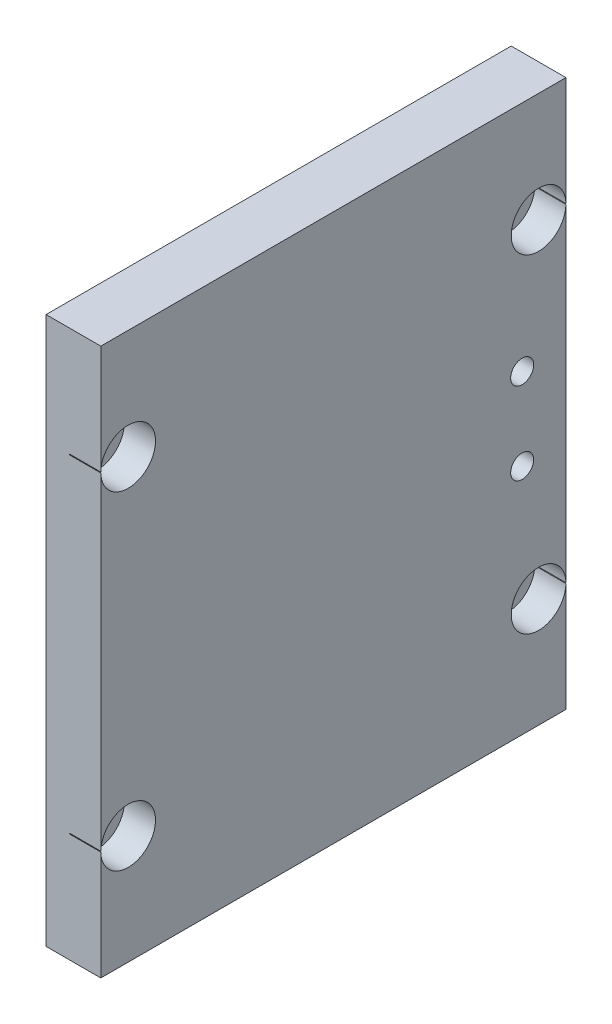
SolidWorks part; units mm, degrees
ref_plane "前视基准面" through (0, 0, 0) normal (0, 0, 1) x (1, 0, 0)
ref_plane "上视基准面" through (0, 0, 0) normal (0, 1, 0) x (1, 0, 0)
ref_plane "右视基准面" through (0, 0, 0) normal (1, 0, 0) x (0, 0, -1)
sketch "草图1" plane through (0, 0, 0) normal (1, 0, 0) x (0, 0, -1)
  line L1 (-42.5, 50) -> (42.5, 50)
  line L2 (-42.5, 50) -> (-42.5, -50)
  line L3 (-42.5, -50) -> (42.5, -50)
  line L4 (42.5, 50) -> (42.5, -50)
  line L5 (-42.5, 50) -> (42.5, -50) construction
  line L6 (-42.5, -50) -> (42.5, 50) construction
  point P0 (0, 0)
  dimension "D1" = 85
  dimension "D2" = 100
extrude "凸台-拉伸1" add sketch "草图1" along normal blind 10
hole_wizard "打孔尺寸(%根据)内六角圆柱头螺钉的类型1" positions "草图2" profile "草图3" counterbore size "M5" standard "GB" end condition through all
sketch "草图2" plane through (10, 0, 0) normal (1, 0, 0) x (0, 0, -1)
  line L0 (0, 67.5491) -> (0, 0) construction
  line L1 (0, 0) -> (51.1342, 0) construction
  point P0 (-37.5, 30)
  point P2 (-37.5, -30)
  point P4 (37.5, 30)
  point P6 (37.5, -30)
  dimension "D1" = 75
  dimension "D2" = 60
sketch "草图3" plane through (10, 30, 37.5) normal (0, 1, 0) x (0, 0, -1)
  line L0 (0, 0) -> (0, 10)
  line L1 (0, 10) -> (2.75, 10)
  line L3 (2.75, 10) -> (2.75, 5.7)
  line L4 (2.75, 5.7) -> (5.0005, 5.7)
  line L5 (5.0005, 5.7) -> (5.0005, 0)
  line L7 (5.0005, 0) -> (0, 0)
  line L11 (0, -6.35) -> (0, 107.95) construction
  dimension "通孔孔直径" = 5.5
  dimension "通孔孔深度" = 10
  dimension "柱形沉头孔直径" = 10.001
  dimension "柱形沉头孔深度" = 5.7
hole_wizard "M5 螺纹孔1" positions "草图4" profile "草图5" tap size "M5" standard "GB" end condition through all
sketch "草图4" plane through (10, 0, 0) normal (1, 0, 0) x (0, 0, -1)
  line L0 (0, 0) -> (63.2893, 0) construction
  line L2 (42.5, -29.9293) -> (42.5, 29.9293) construction
  point P0 (34.5, 7.5)
  point P2 (34.5, -7.5)
  dimension "D1" = 15
  dimension "D2" = 8
sketch "草图5" plane through (10, 7.5, -34.5) normal (0, 1, 0) x (0, 0, -1)
  line L0 (0, 0) -> (0, 10)
  line L1 (0, 10) -> (2.1, 10)
  line L2 (2.1, 10) -> (2.1, 0)
  line L5 (2.1, 0) -> (0, 0)
  line L11 (0, -6.35) -> (0, 107.95) construction
  dimension "通孔螺纹孔钻头直径" = 4.2
  dimension "通孔螺纹孔钻头深度" = 10
cosmetic thread "孔螺蚊线1" parameters "D2"=5
cosmetic thread "孔螺蚊线2" parameters "D2"=5
